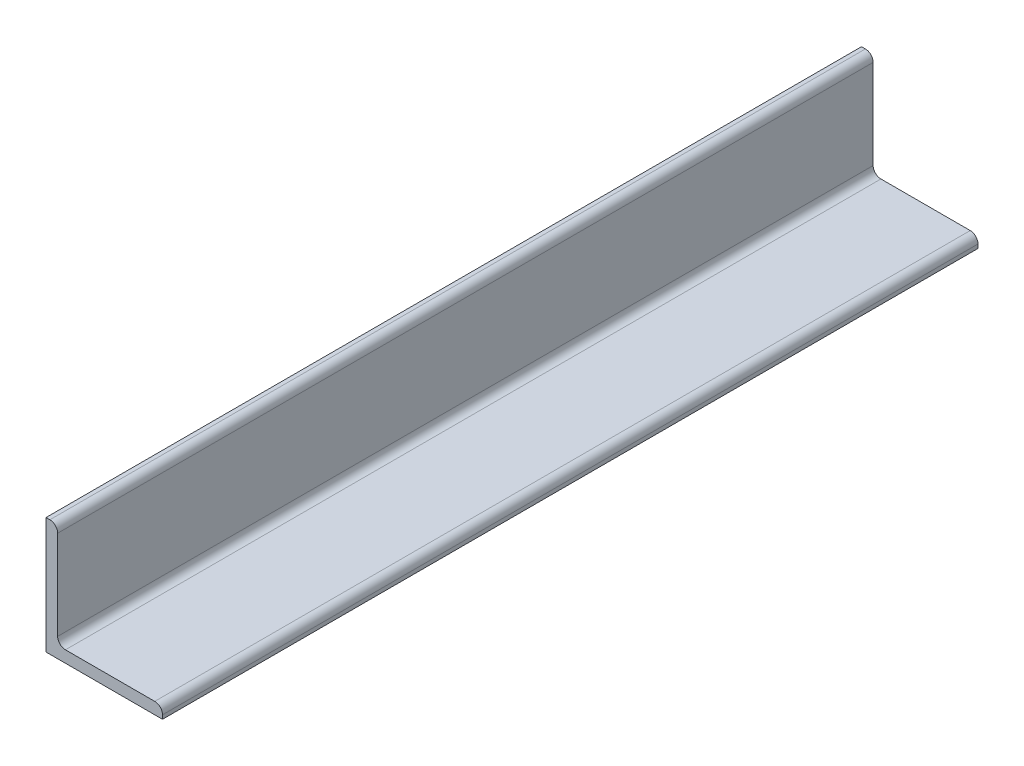
from build123d import *

# Parameters (mm, degrees)
BOSS_EXTRUDE1_DEPTH = 210


with BuildPart() as part:
    # Sketch1 → Boss-Extrude1 (new body)
    with BuildSketch(Plane.XY):
        with BuildLine():
            Line((0, 0), (30, 0))
            Line((30, 0), (30, 1))
            ThreePointArc((30, 1), (29.414213562, 2.414213562), (28, 3))
            Line((28, 3), (5, 3))
            ThreePointArc((5, 3), (3.585786438, 3.585786438), (3, 5))
            Line((3, 5), (3, 28))
            ThreePointArc((3, 28), (2.414213562, 29.414213562), (1, 30))
            Line((1, 30), (0, 30))
            Line((0, 30), (0, 0))
        make_face()
    extrude(amount=BOSS_EXTRUDE1_DEPTH)


solid = part.part
